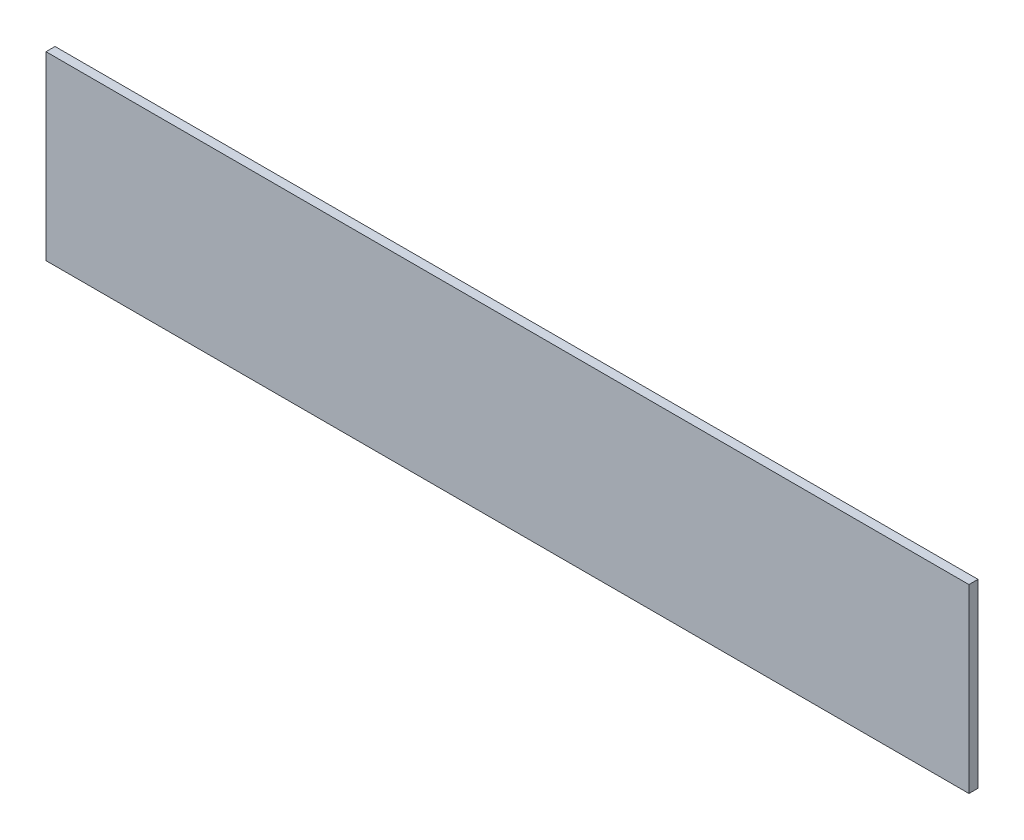
from build123d import *

# Parameters (mm, degrees)
SKETCH1_W           = 510
SKETCH1_H           = 100
BOSS_EXTRUDE1_DEPTH = 5


with BuildPart() as part:
    # Sketch1 → Boss-Extrude1 (new body)
    with BuildSketch(Plane.XY):
        with Locations((255, 50)):
            Rectangle(SKETCH1_W, SKETCH1_H)
    extrude(amount=BOSS_EXTRUDE1_DEPTH)


solid = part.part
